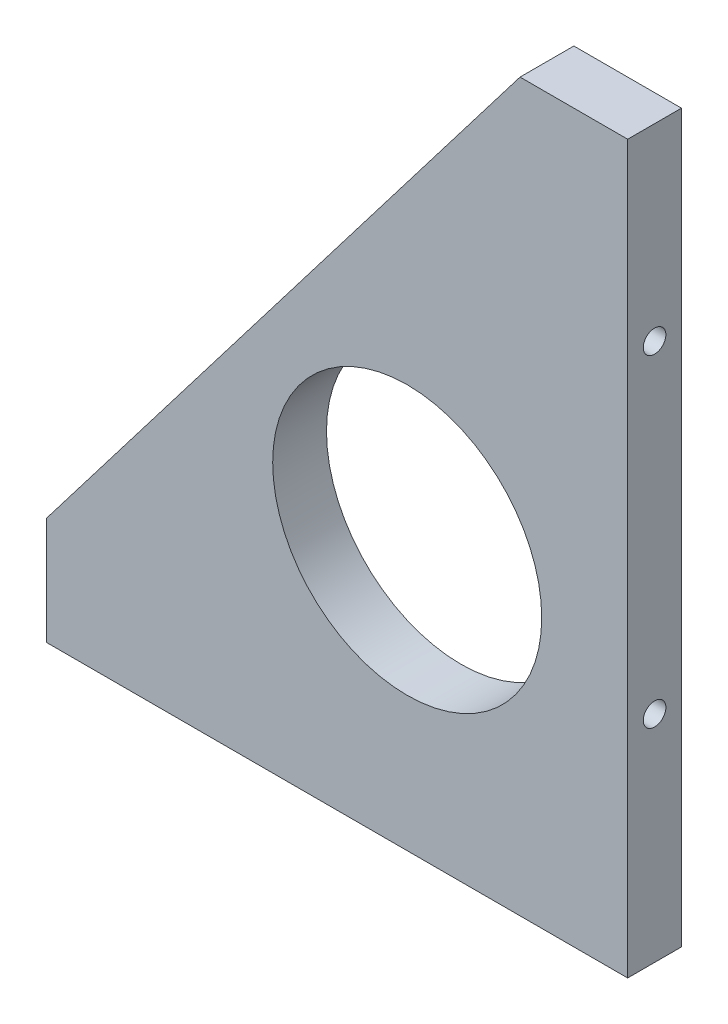
SolidWorks part; units mm, degrees
ref_plane "前视基准面" through (0, 0, 0) normal (0, 0, 1) x (1, 0, 0)
ref_plane "上视基准面" through (0, 0, 0) normal (0, 1, 0) x (1, 0, 0)
ref_plane "右视基准面" through (0, 0, 0) normal (1, 0, 0) x (0, 0, -1)
sketch "草图1" plane through (0, 0, 0) normal (0, 0, 1) x (1, 0, 0)
  line L1 (54, -67.5) -> (-54, -67.5)
  line L2 (54, -67.5) -> (54, 67.5)
  line L3 (54, 67.5) -> (-54, 67.5)
  line L4 (-54, -67.5) -> (-54, 67.5)
  line L5 (54, -67.5) -> (-54, 67.5) construction
  line L6 (54, 67.5) -> (-54, -67.5) construction
  point P0 (0, 0)
  dimension "D1" = 135
  dimension "D2" = 108
extrude "凸台-拉伸1" add sketch "草图1" along normal blind 10
sketch "草图2" plane through (0, 0, 10) normal (0, 0, 1) x (1, 0, 0)
  line L0 (34, 67.5) -> (-54, 67.5)
  line L1 (54, 67.5) -> (-54, 67.5) construction
  line L2 (-54, 67.5) -> (-54, -47.5)
  line L3 (-54, 67.5) -> (-54, -67.5) construction
  line L4 (-54, -47.5) -> (34, 67.5)
  line L5 (54, -67.5) -> (54, 67.5) construction
  line L6 (-54, -67.5) -> (54, -67.5) construction
  dimension "D1" = 20
  dimension "D2" = 20
extrude "切除-拉伸1" cut sketch "草图2" against normal up to next
hole_wizard "M5 螺纹孔1" positions "草图3" profile "草图4" tap size "M5" standard "GB"
sketch "草图3" plane through (0, -67.5, 0) normal (0, -1, 0) x (-1, 0, 0)
  line L0 (-54, -5) -> (-24, -5) construction
  line L1 (-54, -10) -> (-54, 0) construction
  line L2 (-24, -5) -> (26, -5) construction
  point P0 (-24, -5)
  point P2 (26, -5)
  dimension "D1" = 30
  dimension "D2" = 50
sketch "草图4" plane through (24, -67.5, 5) normal (1, 0, 0) x (0, 0, -1)
  line L0 (0, 0) -> (0, 13.6618)
  line L1 (0, 13.6618) -> (2.1, 12.4)
  line L2 (2.1, 12.4) -> (2.1, 0)
  line L5 (2.1, 0) -> (0, 0)
  line L10 (0, 13.6618) -> (-2.1, 12.4) construction
  line L11 (0, -6.35) -> (0, 107.95) construction
  dimension "螺纹孔钻头直径" = 4.2
  dimension "螺纹孔钻头深度" = 12.4
  dimension "导头角度" = 118
cosmetic thread "孔螺蚊线1" parameters "D1"=10, "D2"=5
cosmetic thread "孔螺蚊线2" parameters "D1"=10, "D2"=5
hole_wizard "M5 螺纹孔2" positions "草图5" profile "草图6" tap size "M5" standard "GB"
sketch "草图5" plane through (54, 0, 0) normal (1, 0, 0) x (0, 0, -1)
  line L0 (-5, -67.5) -> (-5, -27.5) construction
  line L1 (-10, -67.5) -> (0, -67.5) construction
  line L2 (-5, -27.5) -> (-5, 32.5) construction
  point P0 (-5, -27.5)
  point P2 (-5, 32.5)
  dimension "D1" = 40
  dimension "D2" = 60
sketch "草图6" plane through (54, -27.5, 5) normal (0, 1, 0) x (0, 0, -1)
  line L0 (0, 0) -> (0, 13.6618)
  line L1 (0, 13.6618) -> (2.1, 12.4)
  line L2 (2.1, 12.4) -> (2.1, 0)
  line L5 (2.1, 0) -> (0, 0)
  line L10 (0, 13.6618) -> (-2.1, 12.4) construction
  line L11 (0, -6.35) -> (0, 107.95) construction
  dimension "螺纹孔钻头直径" = 4.2
  dimension "螺纹孔钻头深度" = 12.4
  dimension "导头角度" = 118
cosmetic thread "孔螺蚊线3" parameters "D1"=10, "D2"=5
cosmetic thread "孔螺蚊线4" parameters "D1"=10, "D2"=5
sketch "草图7" plane through (0, 0, 0) normal (0, 0, -1) x (-1, 0, 0)
  line L0 (14.7675, 3.7697) -> (-13.0281, -17.5) construction
  line L1 (-34, 67.5) -> (54, -47.5) construction
  line L2 (54, -67.5) -> (-54, -67.5) construction
  circle A0 centre (-13.0281, -17.5) radius 25
  dimension "D1" = 50
  dimension "D3" = 50
  dimension "D2" = 35
extrude "切除-拉伸2" cut sketch "草图7" against normal up to next
